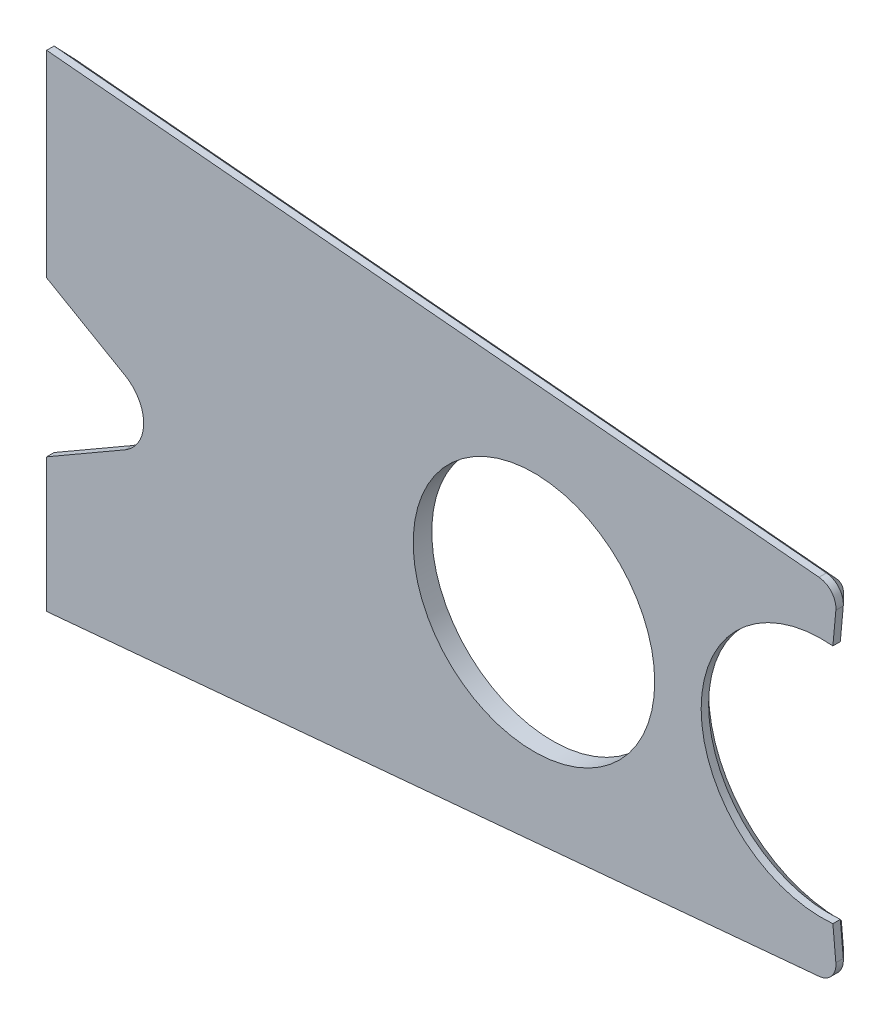
from build123d import *

# Parameters (mm, degrees)
SKETCH1_R           = 65
BOSS_EXTRUDE1_DEPTH = 10
CHAMFER1_SIZE       = 6


with BuildPart() as part:
    # Sketch1 → Boss-Extrude1 (new body)
    with BuildSketch(Plane.XY):
        with BuildLine():
            Line((-262.3, 130.8), (-262.3, 24.7))
            Line((-262.3, 24.7), (-220.073481324, 0.320508076))
            ThreePointArc((-220.073481324, 0.320508076), (-210.073481324, -17), (-220.073481324, -34.320508076))
            Line((-220.073481324, -34.320508076), (-262.3, -58.7))
            Line((-262.3, -58.7), (-262.3, -130.8))
            Line((-262.3, -130.8), (153.441030377, -93.022753927))
            ThreePointArc((153.441030377, -93.022753927), (160.218033303, -89.465947057), (162.495055771, -82.158840075))
            Line((162.495055771, -82.158840075), (160.91140277, -64.73063662))
            ThreePointArc((160.91140277, -64.73063662), (90, 0), (160.91140277, 64.73063662))
            Line((160.91140277, 64.73063662), (162.495055771, 82.158840075))
            ThreePointArc((162.495055771, 82.158840075), (160.218033303, 89.465947057), (153.441030377, 93.022753927))
            Line((153.441030377, 93.022753927), (-262.3, 130.8))
        make_face()
        Circle(SKETCH1_R, mode=Mode.SUBTRACT)
    extrude(amount=BOSS_EXTRUDE1_DEPTH)

    # Chamfer1
    chamfer1_edges = [part.edges().sort_by_distance(p)[0] for p in [
        (-241.186740662, -46.510254038, 0),
        (-210.073481324, -17, 0),
        (-241.186740662, 12.510254038, 0),
        (-262.3, 77.75, 0),
        (-54.429484811, 111.911376963, 0),
        (160.218033303, 89.465947057, 0),
        (161.703229271, 73.444738348, 0),
        (90, 0, 0),
        (161.703229271, -73.444738348, 0),
        (160.218033303, -89.465947057, 0),
        (-54.429484811, -111.911376963, 0),
        (-262.3, -94.75, 0),
    ]]
    chamfer(chamfer1_edges, length=CHAMFER1_SIZE)


solid = part.part
